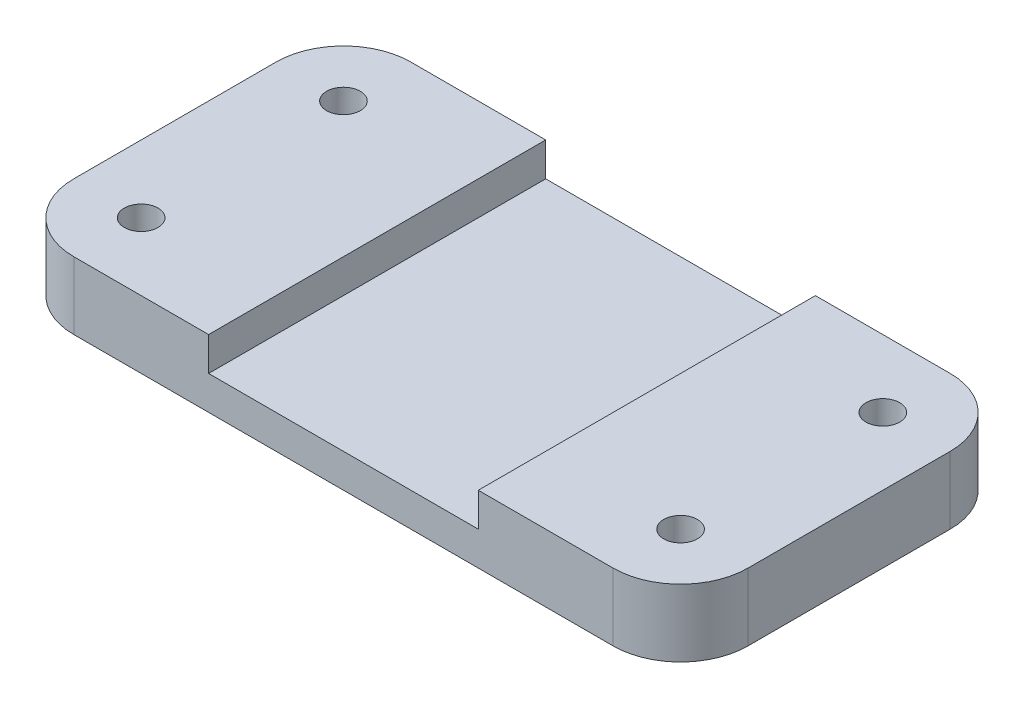
from build123d import *

# Parameters (mm, degrees)
SKETCH1_W             = 100
SKETCH1_H             = 50
BOSS_EXTRUDE1_DEPTH   = 10
FILLET1_R             = 10
M6_TAPPED_HOLE1_D     = 5
M6_TAPPED_HOLE1_DEPTH = 13.497848452
M6_TAPPED_HOLE1_TIP   = 1.502151548
SKETCH2_W             = 40
SKETCH2_H             = 50
CUT_EXTRUDE1_DEPTH    = 5


with BuildPart() as part:
    # Sketch1 → Boss-Extrude1 (new body)
    with BuildSketch(Plane(origin=(0, 0, 0), x_dir=(1, 0, 0), z_dir=(0, 1, 0))):
        Rectangle(SKETCH1_W, SKETCH1_H)
    extrude(amount=BOSS_EXTRUDE1_DEPTH)

    # Fillet1
    fillet1_edges = [part.edges().sort_by_distance(p)[0] for p in [
        (50, 5, 25),
        (-50, 5, 25),
        (-50, 5, -25),
        (50, 5, -25),
    ]]
    fillet(fillet1_edges, radius=FILLET1_R)

    # M6 Tapped Hole1
    with Locations(Plane(origin=(-40, 10, 15), x_dir=(0, 0, 1), z_dir=(0, 1, 0))):
        with Locations((0, 0), (-30, 0), (-30, 80), (0, 80)):
            Hole(M6_TAPPED_HOLE1_D / 2, depth=M6_TAPPED_HOLE1_DEPTH)
            with Locations((0, 0, -(M6_TAPPED_HOLE1_DEPTH + M6_TAPPED_HOLE1_TIP / 2))):  # 118° drill point
                Cone(0, M6_TAPPED_HOLE1_D / 2, M6_TAPPED_HOLE1_TIP, mode=Mode.SUBTRACT)

    # Sketch2 → Cut-Extrude1 (cut)
    with BuildSketch(Plane(origin=(0, 10, 0), x_dir=(1, 0, 0), z_dir=(0, 1, 0))):
        Rectangle(SKETCH2_W, SKETCH2_H)
    extrude(amount=-CUT_EXTRUDE1_DEPTH, mode=Mode.SUBTRACT)


solid = part.part
